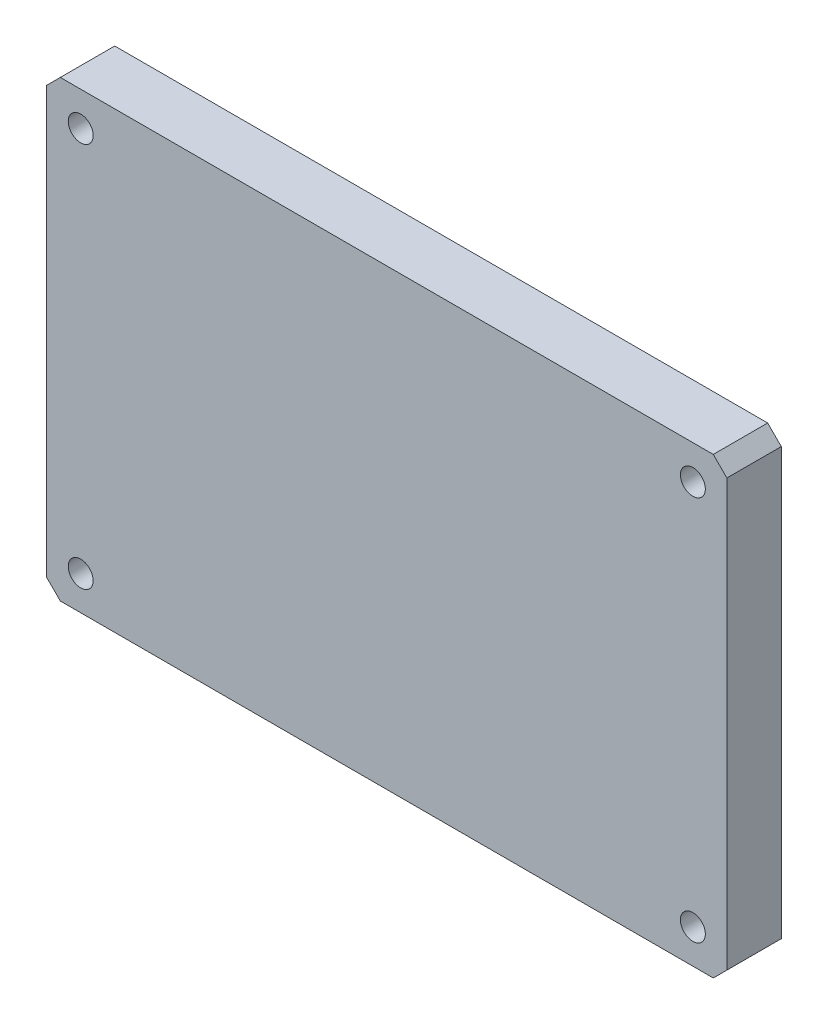
SolidWorks part; units mm, degrees
ref_plane "Front Plane" through (0, 0, 0) normal (0, 0, 1) x (1, 0, 0)
ref_plane "Top Plane" through (0, 0, 0) normal (0, 1, 0) x (1, 0, 0)
ref_plane "Right Plane" through (0, 0, 0) normal (1, 0, 0) x (0, 0, -1)
sketch "Sketch1" plane through (0, 0, 0) normal (0, 0, 1) x (1, 0, 0)
  line L1 (-75, -50) -> (75, -50)
  line L2 (-75, -50) -> (-75, 50)
  line L3 (-75, 50) -> (75, 50)
  line L4 (75, -50) -> (75, 50)
  line L5 (-75, -50) -> (75, 50) construction
  line L6 (-75, 50) -> (75, -50) construction
  point P0 (0, 0)
  dimension "D1" = 150
  dimension "D2" = 100
extrude "Boss-Extrude1" add sketch "Sketch1" along normal blind 12
sketch "Sketch5" plane through (0, 0, 0) normal (0, 0, -1) x (-1, 0, 0)
  line L0 (-56.0087, -40.6513) -> (-56.0087, -24.0513)
  line L1 (-56.2087, -23.8513) -> (-64.8087, -23.8513)
  line L2 (-65.0087, -23.6513) -> (-65.0087, -17.6513)
  line L3 (-64.8087, -17.4513) -> (-60.6087, -17.4513)
  line L4 (-60.4087, -17.2513) -> (-60.4087, 4.9487)
  line L5 (-60.6087, 5.1487) -> (-64.8087, 5.1487)
  line L6 (-65.0087, 5.3487) -> (-65.0087, 11.3487)
  line L7 (-64.8087, 11.5487) -> (-59.2087, 11.5487)
  line L8 (-59.0087, 11.7487) -> (-59.0087, 36.2487)
  line L9 (-58.8087, 36.4487) -> (-43.7087, 36.4487)
  line L10 (-43.5087, 36.6487) -> (-43.5087, 39.6487)
  line L11 (-43.3087, 39.8487) -> (-37.3087, 39.8487)
  line L12 (-37.1087, 39.6487) -> (-37.1087, 36.6487)
  line L13 (-36.9087, 36.4487) -> (-4.7087, 36.4487)
  line L14 (-4.5087, 36.6487) -> (-4.5087, 39.6487)
  line L15 (-4.3087, 39.8487) -> (1.6913, 39.8487)
  line L16 (1.8913, 39.6487) -> (1.8913, 36.6487)
  line L17 (2.0913, 36.4487) -> (40.2913, 36.4487)
  line L18 (40.4913, 36.6487) -> (40.4913, 39.6487)
  line L19 (40.6913, 39.8487) -> (46.6913, 39.8487)
  line L20 (46.8913, 39.6487) -> (46.8913, 36.6487)
  line L21 (47.0913, 36.4487) -> (62.1913, 36.4487)
  line L22 (62.3913, 36.2487) -> (62.3913, 11.7487)
  line L23 (62.5913, 11.5487) -> (68.1913, 11.5487)
  line L24 (68.3913, 11.3487) -> (68.3913, 5.3487)
  line L25 (68.1913, 5.1487) -> (62.5913, 5.1487)
  line L26 (62.3913, 4.9487) -> (62.3913, -17.2513)
  line L27 (62.5913, -17.4513) -> (68.1913, -17.4513)
  line L28 (68.3913, -17.6513) -> (68.3913, -23.6513)
  line L29 (68.1913, -23.8513) -> (59.5913, -23.8513)
  line L30 (59.3913, -24.0513) -> (59.3913, -40.6513)
  line L31 (59.1913, -40.8513) -> (-55.8087, -40.8513)
  arc A0 (-55.8087, -40.8513) -> (-56.0087, -40.6513) centre (-55.8087, -40.6513) cw
  arc A1 (59.3913, -40.6513) -> (59.1913, -40.8513) centre (59.1913, -40.6513) cw
  arc A2 (68.3913, -23.6513) -> (68.1913, -23.8513) centre (68.1913, -23.6513) cw
  arc A3 (68.1913, -17.4513) -> (68.3913, -17.6513) centre (68.1913, -17.6513) cw
  arc A4 (59.5913, -23.8513) -> (59.3913, -24.0513) centre (59.5913, -24.0513) ccw
  arc A5 (62.5913, 5.1487) -> (62.3913, 4.9487) centre (62.5913, 4.9487) ccw
  arc A6 (68.3913, 5.3487) -> (68.1913, 5.1487) centre (68.1913, 5.3487) cw
  arc A7 (68.1913, 11.5487) -> (68.3913, 11.3487) centre (68.1913, 11.3487) cw
  arc A8 (62.3913, 11.7487) -> (62.5913, 11.5487) centre (62.5913, 11.7487) ccw
  arc A9 (46.8913, 36.6487) -> (47.0913, 36.4487) centre (47.0913, 36.6487) ccw
  arc A10 (62.3913, -17.2513) -> (62.5913, -17.4513) centre (62.5913, -17.2513) ccw
  arc A11 (46.6913, 39.8487) -> (46.8913, 39.6487) centre (46.6913, 39.6487) cw
  arc A12 (40.4913, 39.6487) -> (40.6913, 39.8487) centre (40.6913, 39.6487) cw
  arc A13 (1.8913, 36.6487) -> (2.0913, 36.4487) centre (2.0913, 36.6487) ccw
  arc A14 (40.2913, 36.4487) -> (40.4913, 36.6487) centre (40.2913, 36.6487) ccw
  arc A15 (1.6913, 39.8487) -> (1.8913, 39.6487) centre (1.6913, 39.6487) cw
  arc A16 (-4.5087, 39.6487) -> (-4.3087, 39.8487) centre (-4.3087, 39.6487) cw
  arc A17 (-4.7087, 36.4487) -> (-4.5087, 36.6487) centre (-4.7087, 36.6487) ccw
  arc A18 (-37.1087, 36.6487) -> (-36.9087, 36.4487) centre (-36.9087, 36.6487) ccw
  arc A19 (-37.3087, 39.8487) -> (-37.1087, 39.6487) centre (-37.3087, 39.6487) cw
  arc A20 (-43.5087, 39.6487) -> (-43.3087, 39.8487) centre (-43.3087, 39.6487) cw
  arc A21 (-43.7087, 36.4487) -> (-43.5087, 36.6487) centre (-43.7087, 36.6487) ccw
  arc A22 (-59.0087, 36.2487) -> (-58.8087, 36.4487) centre (-58.8087, 36.2487) cw
  arc A23 (-59.2087, 11.5487) -> (-59.0087, 11.7487) centre (-59.2087, 11.7487) ccw
  arc A24 (-65.0087, 11.3487) -> (-64.8087, 11.5487) centre (-64.8087, 11.3487) cw
  arc A25 (-64.8087, 5.1487) -> (-65.0087, 5.3487) centre (-64.8087, 5.3487) cw
  arc A26 (-60.4087, 4.9487) -> (-60.6087, 5.1487) centre (-60.6087, 4.9487) ccw
  arc A27 (-60.6087, -17.4513) -> (-60.4087, -17.2513) centre (-60.6087, -17.2513) ccw
  arc A28 (-65.0087, -17.6513) -> (-64.8087, -17.4513) centre (-64.8087, -17.6513) cw
  arc A29 (-64.8087, -23.8513) -> (-65.0087, -23.6513) centre (-64.8087, -23.6513) cw
  arc A30 (62.1913, 36.4487) -> (62.3913, 36.2487) centre (62.1913, 36.2487) cw
  arc A31 (-56.0087, -24.0513) -> (-56.2087, -23.8513) centre (-56.2087, -24.0513) ccw
  dimension "D33" = 0.2
extrude "Cut-Extrude3" cut sketch "Sketch5" against normal blind 1
chamfer "Chamfer1" distance 3 angle 45 4 edges at (-75, 50, 6) (-75, -50, 6) (75, 50, 6) (75, -50, 6)
hole_wizard "Hole Size (%based) Socket Head Cap Screw Type1" positions "Sketch6" profile "Sketch7" counterbore size "M5" standard "GB" end condition through all
sketch "Sketch6" plane through (0, 0, 0) normal (0, 0, -1) x (-1, 0, 0)
  line L0 (0, 0) -> (50000, 0) construction
  line L1 (0, 0) -> (0, -50000) construction
  line L2 (-72, 50) -> (72, 50) construction
  line L3 (-75, -47) -> (-75, 47) construction
  point P0 (-67.5, 42.5)
  point P9 (67.5, 42.5)
  point P10 (67.5, -42.5)
  point P11 (-67.5, -42.5)
  dimension "D1" = 7.5
  dimension "D2" = 7.5
sketch "Sketch7" plane through (67.5, 42.5, 0) normal (1, 0, 0) x (0, 1, 0)
  line L0 (0, 0) -> (0, 12)
  line L1 (0, 12) -> (2.75, 12)
  line L3 (2.75, 12) -> (2.75, 5.7)
  line L4 (2.75, 5.7) -> (5, 5.7)
  line L5 (5, 5.7) -> (5, 0)
  line L7 (5, 0) -> (0, 0)
  line L11 (0, -6.35) -> (0, 107.95) construction
  dimension "通孔孔直径" = 5.5
  dimension "通孔孔深度" = 12
  dimension "柱形沉头孔直径" = 10
  dimension "柱形沉头孔深度" = 5.7
